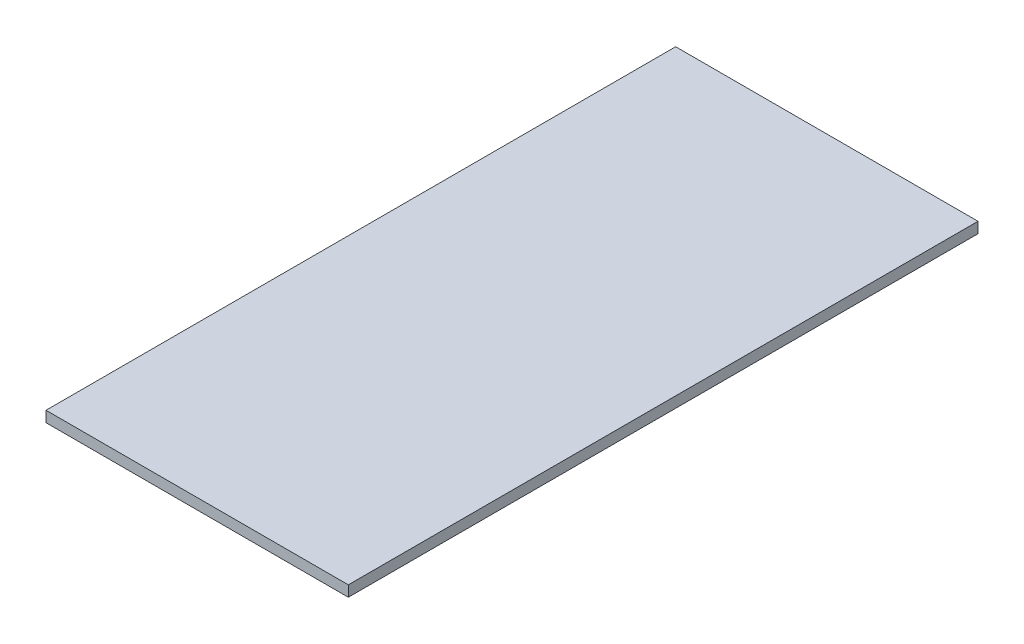
SolidWorks part; units mm, degrees
ref_plane "前视基准面" through (0, 0, 0) normal (0, 0, 1) x (1, 0, 0)
ref_plane "上视基准面" through (0, 0, 0) normal (0, 1, 0) x (1, 0, 0)
ref_plane "右视基准面" through (0, 0, 0) normal (1, 0, 0) x (0, 0, -1)
sketch "草图1" plane through (0, 0, 0) normal (0, 1, 0) x (1, 0, 0)
  line L0 (0, 0) -> (840.28, 0)
  line L1 (840.28, 0) -> (840.28, -1750)
  line L2 (840.28, -1750) -> (0, -1750)
  line L3 (0, -1750) -> (0, 0)
extrude "凸台-拉伸1" add sketch "草图1" along normal blind 30
